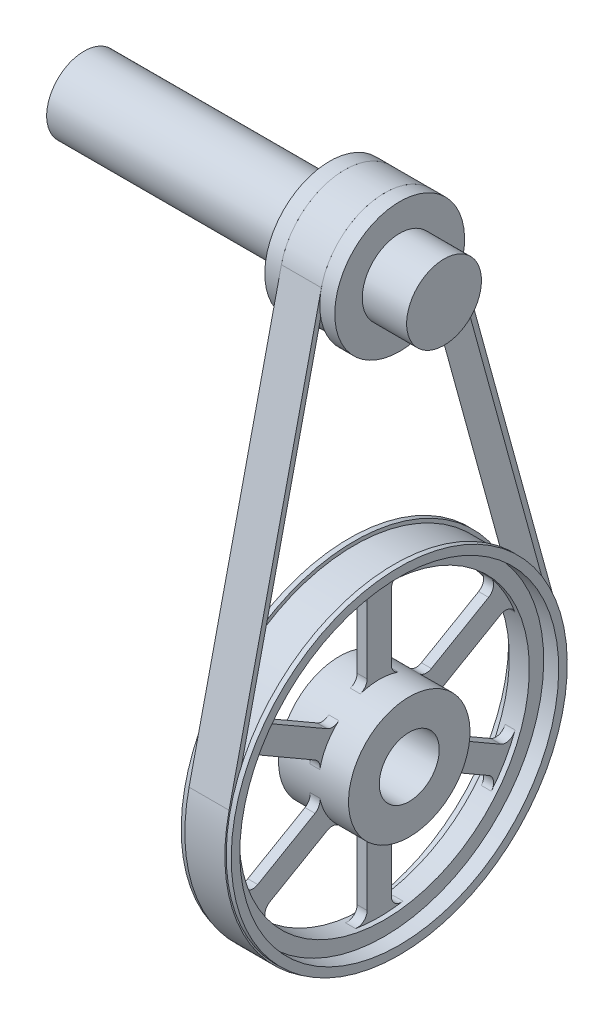
from build123d import *

# Parameters (mm, degrees)
SKETCH2_R                = 6.074823011
SKETCH2_R_2              = 3
BOSS_EXTRUDE1_DEPTH      = 7
SKETCH3_R                = 16.806364111
SKETCH3_R_2              = 15.947327111
BOSS_EXTRUDE2_DEPTH      = 2.5
SKETCH4_R                = 15.947327111
SKETCH4_R_2              = 14.512031262
BOSS_EXTRUDE3_DEPTH      = 1
BOSS_EXTRUDE4_DEPTH      = 0.5
FILLET1_R                = 1
FILLET2_R                = 1
SKETCH6_R                = 19.088387017
SKETCH6_R_2              = 16.442182257
CUT_EXTRUDE1_DEPTH       = 2
BOSS_EXTRUDE5_DEPTH      = 32
BOSS_EXTRUDE5_DEPTH_BACK = 4
SKETCH7_R                = 3.742217825
SKETCH8_R                = 6.491949868
SKETCH8_R_2              = 3.742217825
BOSS_EXTRUDE6_DEPTH      = 7
SKETCH9_R                = 7.17344487
SKETCH9_R_2              = 5.997832818
CUT_EXTRUDE2_DEPTH       = 2
BOSS_EXTRUDE7_DEPTH      = 4


with BuildPart() as part:
    # Sketch2 → Boss-Extrude1 (new body)
    with BuildSketch(Plane.ZY.offset(-54.999571017)):
        with Locations(Location((-0.957893929, -42.45948374, 0), (0, 0, 270))):
            Circle(SKETCH2_R)
        with Locations(Location((-0.957893929, -42.45948374, 0), (0, 0, 270))):
            Circle(SKETCH2_R_2, mode=Mode.SUBTRACT)
    extrude(amount=-BOSS_EXTRUDE1_DEPTH)



with BuildPart() as body_2:
    # Sketch3 → Boss-Extrude2 (new, symmetric)
    with BuildSketch(Plane.ZY.offset(-58.499571017)):
        with Locations(Location((-0.957893929, -42.45948374, 0), (0, 0, 270))):
            Circle(SKETCH3_R)
        with Locations(Location((-0.957893929, -42.45948374, 0), (0, 0, 270))):
            Circle(SKETCH3_R_2, mode=Mode.SUBTRACT)
    extrude(amount=BOSS_EXTRUDE2_DEPTH, both=True)

    # Sketch4 → Boss-Extrude3 (add, symmetric)
    with BuildSketch(Plane.ZY.offset(-58.499571017)):
        with Locations(Location((-0.957893929, -42.45948374, 0), (0, 0, 270))):
            Circle(SKETCH4_R)
        with Locations(Location((-0.957893929, -42.45948374, 0), (0, 0, 270))):
            Circle(SKETCH4_R_2, mode=Mode.SUBTRACT)
    extrude(amount=BOSS_EXTRUDE3_DEPTH, both=True)


with BuildPart() as part_1:
    add(part.part)

    add(body_2.part)  # Boss-Extrude4 merges body 2
    # Sketch5 → Boss-Extrude4 (add, symmetric)
    with BuildSketch(Plane.ZY.offset(-58.499571017)):
        with BuildLine():
            Line((10.959248998, -34.178133861), (3.590416559, -38.432531254))
            ThreePointArc((3.590416559, -38.432531254), (4.303057122, -39.422072234), (4.803704468, -40.534007556))
            Line((4.803704468, -40.534007556), (12.172536907, -36.279610164))
            ThreePointArc((12.172536907, -36.279610164), (11.609893805, -35.203468109), (10.959248998, -34.178133861))
        make_face()
        with BuildLine():
            Line((-2.171181838, -27.998260285), (-2.171181838, -36.50705507))
            ThreePointArc((-2.171181838, -36.50705507), (-0.957893929, -36.384660729), (0.25539398, -36.50705507))
            Line((0.25539398, -36.50705507), (0.25539398, -27.998260285))
            ThreePointArc((0.25539398, -27.998260285), (-0.957893929, -27.947452478), (-2.171181838, -27.998260285))
        make_face()
        with BuildLine():
            Line((12.172536907, -48.639357316), (4.803704468, -44.384959923))
            ThreePointArc((4.803704468, -44.384959923), (4.303057122, -45.496895245), (3.590416559, -46.486436226))
            Line((3.590416559, -46.486436226), (10.959248998, -50.740833618))
            ThreePointArc((10.959248998, -50.740833618), (11.609893805, -49.715499371), (12.172536907, -48.639357316))
        make_face()
        with BuildLine():
            Line((0.25539398, -56.920707194), (0.25539398, -48.411912409))
            ThreePointArc((0.25539398, -48.411912409), (-0.957893929, -48.534306751), (-2.171181838, -48.411912409))
            Line((-2.171181838, -48.411912409), (-2.171181838, -56.920707194))
            ThreePointArc((-2.171181838, -56.920707194), (-0.957893929, -56.971515002), (0.25539398, -56.920707194))
        make_face()
        with BuildLine():
            Line((-12.875036856, -50.740833618), (-5.506204416, -46.486436226))
            ThreePointArc((-5.506204416, -46.486436226), (-6.21884498, -45.496895245), (-6.719492325, -44.384959923))
            Line((-6.719492325, -44.384959923), (-14.088324765, -48.639357316))
            ThreePointArc((-14.088324765, -48.639357316), (-13.525681662, -49.715499371), (-12.875036856, -50.740833618))
        make_face()
        with BuildLine():
            Line((-14.088324765, -36.279610164), (-6.719492325, -40.534007556))
            ThreePointArc((-6.719492325, -40.534007556), (-6.21884498, -39.422072234), (-5.506204416, -38.432531254))
            Line((-5.506204416, -38.432531254), (-12.875036856, -34.178133861))
            ThreePointArc((-12.875036856, -34.178133861), (-13.525681662, -35.203468109), (-14.088324765, -36.279610164))
        make_face()
    extrude(amount=BOSS_EXTRUDE4_DEPTH, both=True)

    # Fillet1
    fillet1_edges = [part_1.edges().sort_by_distance(p)[0] for p in [
        (58.499571017, -34.178133861, -12.875036856),
        (58.499571017, -36.279610164, -14.088324765),
        (58.499571017, -40.534007556, -6.719492325),
        (58.499571017, -38.432531254, -5.506204416),
    ]]
    fillet(fillet1_edges, radius=FILLET1_R)

    # Fillet2
    fillet2_edges = [part_1.edges().sort_by_distance(p)[0] for p in [
        (58.499571017, -27.998260285, 0.25539398),
        (58.499571017, -27.998260285, -2.171181838),
        (58.499571017, -36.50705507, -2.171181838),
        (58.499571017, -36.50705507, 0.25539398),
        (58.499571017, -36.279610164, 12.172536907),
        (58.499571017, -34.178133861, 10.959248998),
        (58.499571017, -38.432531254, 3.590416559),
        (58.499571017, -40.534007556, 4.803704468),
        (58.499571017, -50.740833618, 10.959248998),
        (58.499571017, -48.639357316, 12.172536907),
        (58.499571017, -44.384959923, 4.803704468),
        (58.499571017, -46.486436226, 3.590416559),
        (58.499571017, -56.920707194, -2.171181838),
        (58.499571017, -56.920707194, 0.25539398),
        (58.499571017, -48.411912409, 0.25539398),
        (58.499571017, -48.411912409, -2.171181838),
        (58.499571017, -48.639357316, -14.088324765),
        (58.499571017, -50.740833618, -12.875036856),
        (58.499571017, -46.486436226, -5.506204416),
        (58.499571017, -44.384959923, -6.719492325),
    ]]
    fillet(fillet2_edges, radius=FILLET2_R)

    # Sketch6 → Cut-Extrude1 (cut, symmetric)
    with BuildSketch(Plane.ZY.offset(-58.499571017)):
        with Locations((-0.957893929, -42.45948374)):
            Circle(SKETCH6_R)
        with Locations(Location((-0.957893929, -42.45948374, 0), (0, 0, 270))):
            Circle(SKETCH6_R_2, mode=Mode.SUBTRACT)
    extrude(amount=CUT_EXTRUDE1_DEPTH, both=True, mode=Mode.SUBTRACT)


with BuildPart() as body_2_2:
    # Sketch7 → Boss-Extrude5 (new, two sides: drawn at the far end of the back side and taken through both)
    with BuildSketch(Plane(origin=(34.437162011, 0, 0), x_dir=(0, 0, -1), z_dir=(1, 0, 0)).offset(-BOSS_EXTRUDE5_DEPTH_BACK)):
        with Locations((0, 0.49221935)):
            Circle(SKETCH7_R)
    extrude(amount=BOSS_EXTRUDE5_DEPTH + BOSS_EXTRUDE5_DEPTH_BACK)

    # Sketch8 → Boss-Extrude6 (add)
    with BuildSketch(Plane.ZY.offset(-54.999571017)):
        with Locations(Location((0, 0.49221935, 0), (0, 0, 270))):
            Circle(SKETCH8_R)
        with Locations(Location((0, 0.49221935, 0), (0, 0, 180))):
            Circle(SKETCH8_R_2, mode=Mode.SUBTRACT)
    extrude(amount=-BOSS_EXTRUDE6_DEPTH)

    # Sketch9 → Cut-Extrude2 (cut, symmetric)
    with BuildSketch(Plane.ZY.offset(-58.499571017)):
        with Locations((0, 0.49221935)):
            Circle(SKETCH9_R)
        with Locations(Location((0, 0.49221935, 0), (0, 0, 270))):
            Circle(SKETCH9_R_2, mode=Mode.SUBTRACT)
    extrude(amount=CUT_EXTRUDE2_DEPTH, both=True, mode=Mode.SUBTRACT)


with BuildPart() as body_3:
    # Sketch11 → Boss-Extrude7 (new body)
    with BuildSketch(Plane.ZY.offset(-60.499571017)):
        with BuildLine():
            Line((-6.260195764, 2.211336008), (-17.295262478, -37.973067741))
            ThreePointArc((-17.295262478, -37.973067741), (-1.335638653, -59.397454354), (15.56324097, -38.705866646))
            Line((15.56324097, -38.705866646), (6.330611836, 1.9305402))
            ThreePointArc((6.330611836, 1.9305402), (0.144745215, 6.98255539), (-6.260195764, 2.211336008))
        make_face()
        with BuildLine():
            Line((-5.783942204, 2.079673631), (-16.813726321, -38.10770979))
            ThreePointArc((-16.813726321, -38.10770979), (-1.324490599, -58.897578649), (15.076181077, -38.818907402))
            Line((15.076181077, -38.818907402), (5.848962125, 1.820240648))
            ThreePointArc((5.848962125, 1.820240648), (0.133728328, 6.488561171), (-5.783942204, 2.079673631))
        make_face(mode=Mode.SUBTRACT)
    extrude(amount=BOSS_EXTRUDE7_DEPTH)


solid = Compound([part_1.part, body_2_2.part, body_3.part])
